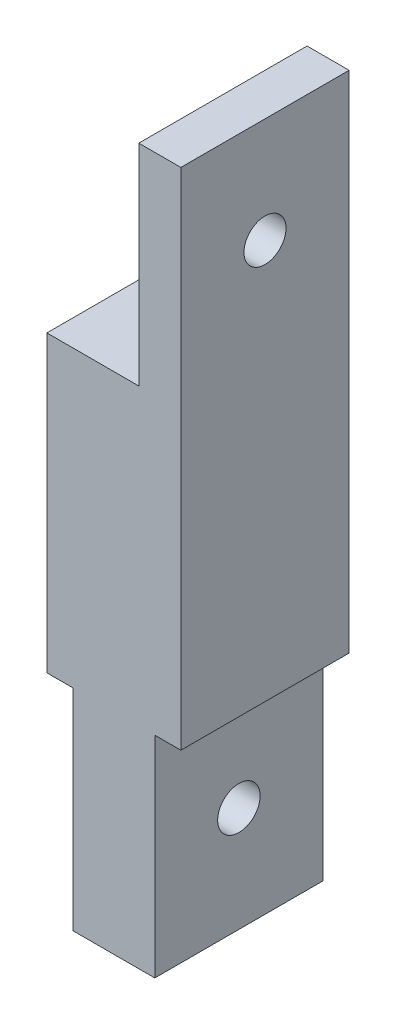
SolidWorks part; units mm, degrees
other "Markup1"
sketch "草图13" plane through (-15.927, 6.82, -43.18) normal (-0.9751, 0.0072, -0.2219) x (-0.2217, -0.0822, 0.9716)
material "PET"
ref_plane "Front Plane" through (0, 0, 0) normal (0, 0, 1) x (1, 0, 0)
ref_plane "Top Plane" through (0, 0, 0) normal (0, 1, 0) x (1, 0, 0)
ref_plane "Right Plane" through (0, 0, 0) normal (1, 0, 0) x (0, 0, -1)
sketch "Sketch1" plane through (0, 0, 0) normal (0, 0, 1) x (1, 0, 0)
  line L0 (-6.35, 0) -> (-6.35, -25.4)
  line L1 (0, 6.35) -> (0, -31.75) construction
  line L2 (0, 6.35) -> (0, -31.75)
  arc A0 (0, 6.35) -> (-6.35, 0) centre (0, 0) ccw
  arc A1 (-6.35, -25.4) -> (0, -31.75) centre (0, -25.4) ccw
  dimension "D1" = 38.1
  dimension "D2" = 6.35
revolve "Revolve1" add sketch "Sketch1" angle 360 about L1
sketch "Sketch2" plane through (0, 0, 0) normal (1, 0, 0) x (0, 0, -1)
  line L0 (2.5, 7.6185) -> (2.5, -6.35)
  line L1 (2.5, -6.35) -> (-2.5, -6.35)
  line L2 (-2.5, -6.35) -> (-2.5, 7.6185)
  line L3 (-2.5, 7.6185) -> (2.5, 7.6185)
  dimension "D1" = 6.35
  dimension "D2" = 5
  dimension "D3" = 2.5
extrude "Cut-Extrude1" cut sketch "Sketch2" against normal through all both and the other way through all
sketch "Sketch3" plane through (0, 0, -2.5) normal (0, 0, 1) x (1, 0, 0)
  circle A0 centre (0, 0) radius 2.54
  dimension "D1" = 5.08
sketch "Sketch4" plane through (0, 0, 0) normal (0, 0, 1) x (1, 0, 0)
  line L0 (2.5, -40.64) -> (2.5, -21.59)
  line L1 (2.5, -21.59) -> (15.2, -21.59)
  line L2 (15.2, -21.59) -> (15.2, -40.64)
  line L3 (15.2, -40.64) -> (2.5, -40.64)
  line L4 (-6.35, -25.4) -> (6.35, -25.4) construction
  line L5 (-2.5, -40.64) -> (-10.9102, -40.64)
  line L6 (-2.5, -40.64) -> (-2.5, -21.59)
  line L7 (-2.5, -21.59) -> (-10.9102, -21.59)
  line L8 (-10.9102, -40.64) -> (-10.9102, -21.59)
  arc A0 (-6.35, -25.4) -> (6.35, -25.4) centre (0, -25.4) ccw construction
  dimension "D1" = 3.81
  dimension "D2" = 19.05
  dimension "D3" = 12.7
  dimension "D4" = 2.5
  dimension "D5" = 5
  dimension "D6" = 3.81
extrude "Cut-Extrude2" cut sketch "Sketch4" against normal through all both and the other way through all
sketch "Sketch5" plane through (2.5, 0, 0) normal (1, 0, 0) x (0, 0, -1)
  circle A0 centre (0, -25.4) radius 2.54
  arc A1 (-5.8372, -25.4) -> (5.8372, -25.4) centre (0, -25.4) ccw construction
  dimension "D1" = 5.08
extrude "Cut-Extrude3" cut sketch "Sketch3" against normal mid plane 25.4
extrude "Cut-Extrude1-T" cut sketch "Sketch5" against normal mid plane 20
sketch "Sketch1-T" plane through (-2.5, 0, 0) normal (-1, 0, 0) x (0, 0, 1)
  line L0 (-5.8372, -21.59) -> (10.2352, -5.5176)
  line L1 (10.2352, -5.5176) -> (10.2352, -22.9556)
  line L2 (10.2352, -22.9556) -> (-5.8372, -21.59)
  line L3 (-5.8372, -21.59) -> (5.8372, -21.59) construction
  dimension "D1" = 45
extrude "Cut-Extrude2-T" cut sketch "Sketch1-T" along normal blind 7.62
mirror "Espelhar1" about plane through (0, 0, 0) normal (1, 0, 0) of "Cut-Extrude2-T"
sketch "Sketch2-T" plane through (0, 0, 0) normal (0, 0, 1) x (1, 0, 0)
  circle A0 centre (0, 0) radius 4
  dimension "D1" = 8
extrude "Cut-Extrude3-T" cut sketch "Sketch2-T" against normal blind 2.54 from offset 5 offset against normal yes
fillet "Filete2" radius 0.1 6 edges at (2.54, 0, -5) (0, 3.9144, -5) (3.9144, -0.4116, -5) (-3.9144, -0.4116, -5) (0, -4, -5) (0.0414, -3.9998, -6.3499)
fillet "Filete3" radius 0.25 12 edges at (6.35, -15.7528, 0) (-6.35, -15.7528, 0) (2.5, -31.2372, 0) (2.5, -23.495, -5.8372) (2.5, -17.6578, 5.8372) (2.5, -15.7528, 0) (2.5, -27.94, 0) (-2.5, -25.4, -2.54) (-2.5, -31.2372, 0) (-2.5, -17.6578, 5.8372) (-2.5, -23.495, -5.8372) (-2.5, -15.7528, 0)
sketch "Sketch3-T" plane through (0, -6.35, 0) normal (0, 1, 0) x (1, 0, 0)
  circle A0 centre (0, 0) radius 6.35 construction
  circle A1 centre (0, 0) radius 6.45
  circle A2 centre (0, 0) radius 6.25
  dimension "D1" = 0.1
  dimension "D2" = 0.1
extrude "Cut-Extrude4-T" cut sketch "Sketch3-T" along normal blind 0.1
sketch "草图1" plane through (0, 0, 2.5) normal (0, 0, -1) x (-1, 0, 0)
  line L1 (-9.1724, -6.35) -> (15.8499, -6.35)
  line L2 (-9.1724, -6.35) -> (-9.1724, 11.7345)
  line L3 (-9.1724, 11.7345) -> (15.8499, 11.7345)
  line L4 (15.8499, -6.35) -> (15.8499, 11.7345)
extrude "切除-拉伸1" cut sketch "草图1" against normal through all both and the other way through all
scale "Scale1" scale about origin uniform scaling yes scale factor 6.8
sketch "草图3" plane through (0, -43.18, 0) normal (0, 1, 0) x (1, 0, 0)
  line L5 (5, -42.8895) -> (-5, -42.8895)
  line L6 (5, -42.8895) -> (5, 42.8895)
  line L7 (5, 42.8895) -> (-5, 42.8895)
  line L8 (-5, -42.8895) -> (-5, 42.8895)
  line L9 (5, -42.8895) -> (-5, 42.8895) construction
  line L10 (5, 42.8895) -> (-5, -42.8895) construction
  circle A1 centre (0, 0) radius 43.18 construction
  point P0 (0, 0)
  dimension "D1" = 10
extrude "Boss-Extrude1" add sketch "草图3" along normal blind 50
sketch "Sketch5-T" plane through (5, 0, 0) normal (1, 0, 0) x (0, 0, -1)
  line L1 (-42.8895, -18.18) -> (42.8895, -18.18) construction
  line L2 (-42.8895, 6.82) -> (-42.8895, -43.18) construction
  line L3 (42.8895, 6.82) -> (42.8895, -43.18) construction
  line L4 (0, -43.18) -> (0, 6.82) construction
  line L5 (42.8895, -43.18) -> (-42.8895, -43.18) construction
  line L6 (-42.8895, 6.82) -> (42.8895, 6.82) construction
  circle A0 centre (0, -18.18) radius 5
  dimension "D1" = 10
extrude "切除-拉伸2" cut sketch "Sketch5-T" against normal through all both and the other way through all
sketch "Sketch6" plane through (17, 0, 0) normal (1, 0, 0) x (0, 0, -1)
  circle A0 centre (0, -172.72) radius 18.972
  circle A1 centre (0, -172.72) radius 5.1
  dimension "D1" = 10.2
extrude "Boss-Extrude2" add sketch "Sketch6" against normal up to surface (34 mm away)
sketch "Sketch7" plane through (0, 0, 0) normal (0, 1, 0) x (1, 0, 0)
  line L1 (-15.927, -46.3514) -> (-61.466, -46.3514)
  line L2 (-15.927, -46.3514) -> (-15.927, 53.3618)
  line L3 (-15.927, 53.3618) -> (-61.466, 53.3618)
  line L4 (-61.466, -46.3514) -> (-61.466, 53.3618)
  line L5 (15.927, -48.7308) -> (70.5175, -48.7308)
  line L6 (15.927, -48.7308) -> (15.927, 53.3618)
  line L7 (15.927, 53.3618) -> (70.5175, 53.3618)
  line L8 (70.5175, -48.7308) -> (70.5175, 53.3618)
extrude "切除-拉伸3" cut sketch "Sketch7" against normal through all both and the other way through all
sketch "Sketch8" plane through (0, -43.18, 0) normal (0, 1, 0) x (1, 0, 0)
  line L0 (5.927, 42.7713) -> (5.927, -42.7713)
  line L2 (15.927, -40.1353) -> (15.927, 40.1353)
  line L3 (5, 42.8895) -> (5, -42.8895)
  line L4 (15.927, -40.1353) -> (15.927, 40.1353)
  arc A2 (5, -42.8895) -> (15.927, -40.1353) centre (0, 0) ccw
  arc A3 (15.927, 40.1353) -> (5, 42.8895) centre (0, 0) ccw
  arc A4 (5.927, -42.7713) -> (15.927, -40.1353) centre (0, 0) ccw
  arc A5 (15.927, 40.1353) -> (5.927, 42.7713) centre (0, 0) ccw
  dimension "D2" = 10
  dimension "D1" = 0
extrude "Boss-Extrude3" add sketch "Sketch8" along normal up to surface (50 mm away)
sketch "Sketch9" plane through (0, -43.18, 0) normal (0, 1, 0) x (1, 0, 0)
  line L4 (-5, 42.8895) -> (-5, -42.8895)
  line L5 (-5, -42.8895) -> (5, -42.8895)
  line L6 (5, -42.8895) -> (5, 42.8895)
  line L7 (5, 42.8895) -> (-5, 42.8895)
  line L8 (-5, 42.8895) -> (-5, -42.8895)
  line L9 (-5, -42.8895) -> (5, -42.8895)
  line L10 (5, -42.8895) -> (5, 42.8895)
  line L11 (5, 42.8895) -> (-5, 42.8895)
  dimension "D1" = 0
sketch "Sketch10" plane through (-5, 0, 0) normal (-1, 0, 0) x (0, 0, 1)
  circle A0 centre (0, -18.18) radius 5
extrude "Cut-Extrude5" cut sketch "Sketch10" along normal through all both and the other way through all
sketch "Sketch11" plane through (0, 0, 0) normal (0, 0, 1) x (1, 0, 0)
  line L0 (-5, -43.18) -> (-15.927, -43.18) construction
  line L1 (-9.1923, -43.18) -> (5.5246, -43.18)
  line L2 (-9.1923, -43.18) -> (-9.1923, 19.2382)
  line L3 (-9.1923, 19.2382) -> (5.5246, 19.2382)
  line L4 (5.5246, -43.18) -> (5.5246, 19.2382)
extrude "Cut-Extrude6" cut sketch "Sketch11" against normal through all both and the other way through all
sketch "Sketch14" plane through (-15.927, 0, 0) normal (-1, 0, 0) x (0, 0, 1)
  line L0 (0, 6.82) -> (0, -163.18) construction
  line L1 (-42.7713, 6.82) -> (42.7713, 6.82) construction
  line L4 (-53.7219, -163.18) -> (81.0541, -163.18)
  line L5 (-53.7219, -163.18) -> (-53.7219, -221.8799)
  line L6 (-53.7219, -221.8799) -> (81.0541, -221.8799)
  line L7 (81.0541, -163.18) -> (81.0541, -221.8799)
  dimension "D1" = 170
extrude "Cut-Extrude7" cut sketch "Sketch14" against normal through all both and the other way through all
sketch "Sketch15" plane through (-15.927, 0, 0) normal (-1, 0, 0) x (0, 0, 1)
  line L0 (0, -18.18) -> (0, -163.18) construction
  line L1 (-40.1353, -163.18) -> (40.1353, -163.18) construction
sketch "Sketch16" plane through (-15.927, 0, 0) normal (-1, 0, 0) x (0, 0, 1)
  line L0 (0, -18.18) -> (0, -163.18) construction
  line L1 (-66.6167, 20.0891) -> (-20, 20.0891)
  line L2 (-66.6167, 20.0891) -> (-66.6167, -199.7574)
  line L3 (-66.6167, -199.7574) -> (-20, -199.7574)
  line L4 (-20, 20.0891) -> (-20, -199.7574)
  line L5 (0, -18.18) -> (0, -140.4794) construction
  line L6 (20, 20.0891) -> (20, -199.7574)
  line L7 (66.6167, -199.7574) -> (20, -199.7574)
  line L8 (66.6167, 20.0891) -> (66.6167, -199.7574)
  line L9 (66.6167, 20.0891) -> (20, 20.0891)
  dimension "D1" = 20
extrude "Cut-Extrude8" cut sketch "Sketch16" against normal through all both and the other way through all
sketch "Sketch17" plane through (0, 0, 20) normal (0, 0, 1) x (1, 0, 0)
  line L0 (0, -163.18) -> (0, -81.0156) construction
  line L5 (15.927, -163.18) -> (-15.927, -163.18) construction
  line L7 (-9.725, -113.18) -> (-32.6946, -113.18)
  line L8 (-9.725, -113.18) -> (-9.725, -175.1477)
  line L9 (-9.725, -175.1477) -> (-32.6946, -175.1477)
  line L10 (-32.6946, -113.18) -> (-32.6946, -175.1477)
  line L11 (9.725, -113.18) -> (29.0966, -113.18)
  line L12 (9.725, -113.18) -> (9.725, -173.5464)
  line L13 (9.725, -173.5464) -> (29.0966, -173.5464)
  line L14 (29.0966, -113.18) -> (29.0966, -173.5464)
  point P16 (0, -122.0978)
  dimension "D1" = 9.725
  dimension "D2" = 50
  dimension "D3" = 50
  dimension "D5" = 9.725
extrude "Cut-Extrude9" cut sketch "Sketch17" against normal through all both and the other way through all
sketch "Sketch18" plane through (9.725, 0, 0) normal (1, 0, 0) x (0, 0, -1)
  line L0 (-20, -138.18) -> (20, -138.18) construction
  line L1 (-20, -163.18) -> (-20, -113.18) construction
  line L2 (20, -113.18) -> (20, -163.18) construction
  line L3 (0, -163.18) -> (0, -113.18) construction
  line L4 (20, -163.18) -> (-20, -163.18) construction
  line L5 (20, -113.18) -> (-20, -113.18) construction
  circle A0 centre (0, -138.18) radius 5.05
  dimension "D1" = 10.1
extrude "Cut-Extrude10" cut sketch "Sketch18" against normal through all both and the other way through all
